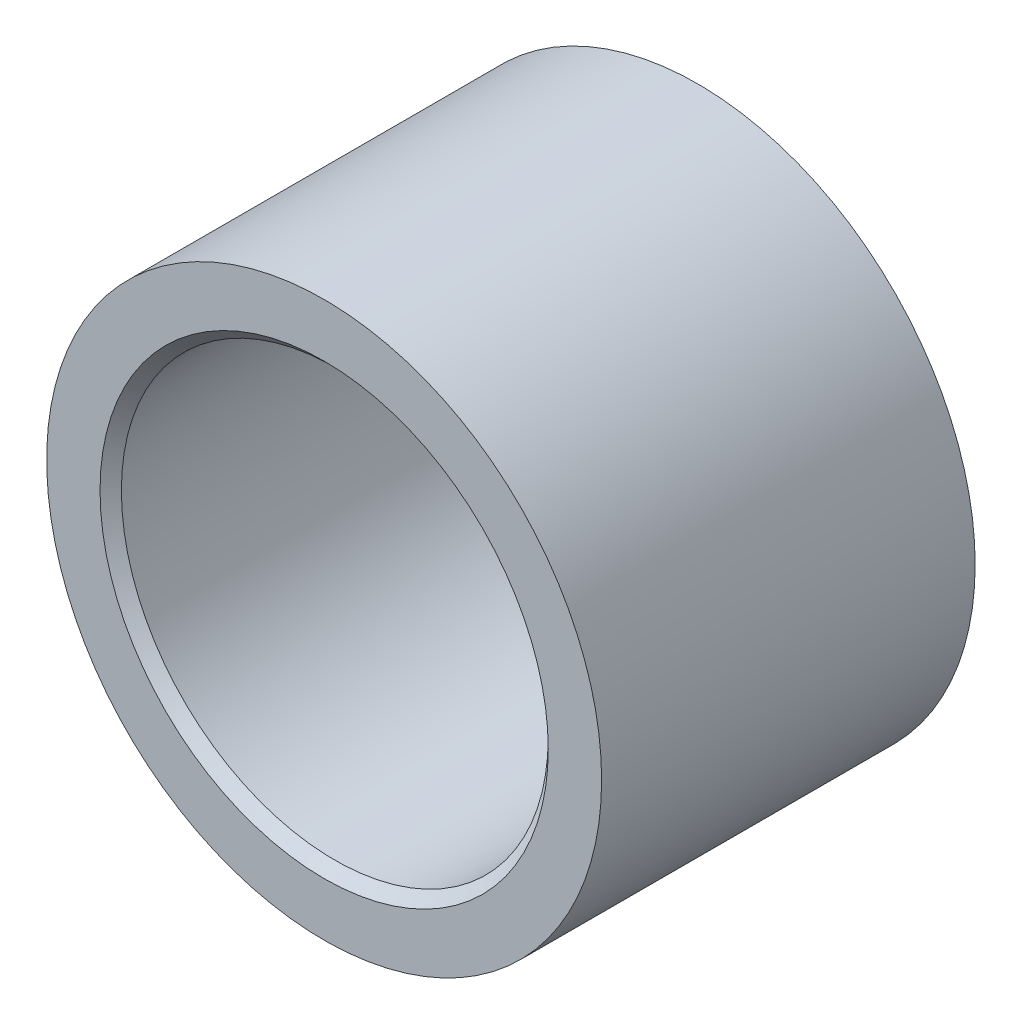
SolidWorks part; units mm, degrees
ref_plane "Front Plane" through (0, 0, 0) normal (0, 0, 1) x (1, 0, 0)
ref_plane "Top Plane" through (0, 0, 0) normal (0, 1, 0) x (1, 0, 0)
ref_plane "Right Plane" through (0, 0, 0) normal (1, 0, 0) x (0, 0, -1)
sketch "Sketch1" plane through (0, 0, 0) normal (0, 0, 1) x (1, 0, 0)
  circle A0 centre (0, 0) radius 10
  circle A1 centre (0, 0) radius 13
  dimension "D1" = 20
  dimension "D2" = 26
extrude "Boss-Extrude1" add sketch "Sketch1" along normal blind 17.5
chamfer "Chamfer1" distance 0.5 angle 45 2 edges at (10, 0, 0) (10, 0, 17.5)
